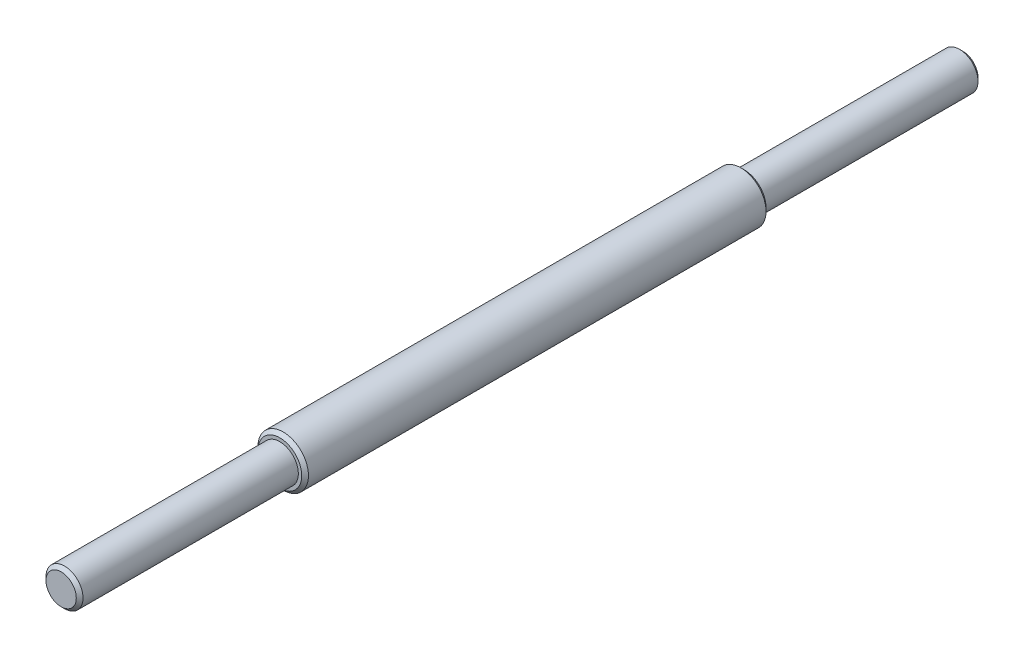
from build123d import *

# Parameters (mm, degrees)
SKETCH1_R           = 7.5
BOSS_EXTRUDE1_DEPTH = 138
SKETCH2_R           = 5.5
BOSS_EXTRUDE2_DEPTH = 20
SKETCH3_R           = 5.5
BOSS_EXTRUDE3_DEPTH = 45
CHAMFER1_SIZE       = 1
BOSS_EXTRUDE4_START = 65
SKETCH4_R           = 5.5
BOSS_EXTRUDE4_DEPTH = 65
CHAMFER2_SIZE       = 1


with BuildPart() as part:
    # Sketch1 → Boss-Extrude1 (new body)
    with BuildSketch(Plane.XY):
        Circle(SKETCH1_R)
    extrude(amount=BOSS_EXTRUDE1_DEPTH)

    # Sketch2 → Boss-Extrude2 (add)
    with BuildSketch(Plane.XY.offset(138)):
        Circle(SKETCH2_R)
    extrude(amount=BOSS_EXTRUDE2_DEPTH)

    # Sketch3 → Boss-Extrude3 (add)
    with BuildSketch(Plane.XY.offset(158)):
        Circle(SKETCH3_R)
    extrude(amount=BOSS_EXTRUDE3_DEPTH)

    # Chamfer1
    chamfer1_edges = [part.edges().sort_by_distance(p)[0] for p in [
        (-7.5, 0, 0),
        (-7.5, 0, 138),
        (-5.5, 0, 203),
    ]]
    chamfer(chamfer1_edges, length=CHAMFER1_SIZE)

    # Sketch4 → Boss-Extrude4 (add)
    with BuildSketch(Plane(origin=(0, 0, 0), x_dir=(-1, 0, 0), z_dir=(0, 0, -1)).offset(BOSS_EXTRUDE4_START)):
        with Locations(Location((0, 0, 0), (0, 0, 180))):
            Circle(SKETCH4_R)
    extrude(amount=-BOSS_EXTRUDE4_DEPTH)

    # Chamfer2
    chamfer2_edges = [part.edges().sort_by_distance(p)[0] for p in [
        (-5.5, 0, -65),
    ]]
    chamfer(chamfer2_edges, length=CHAMFER2_SIZE)


solid = part.part
